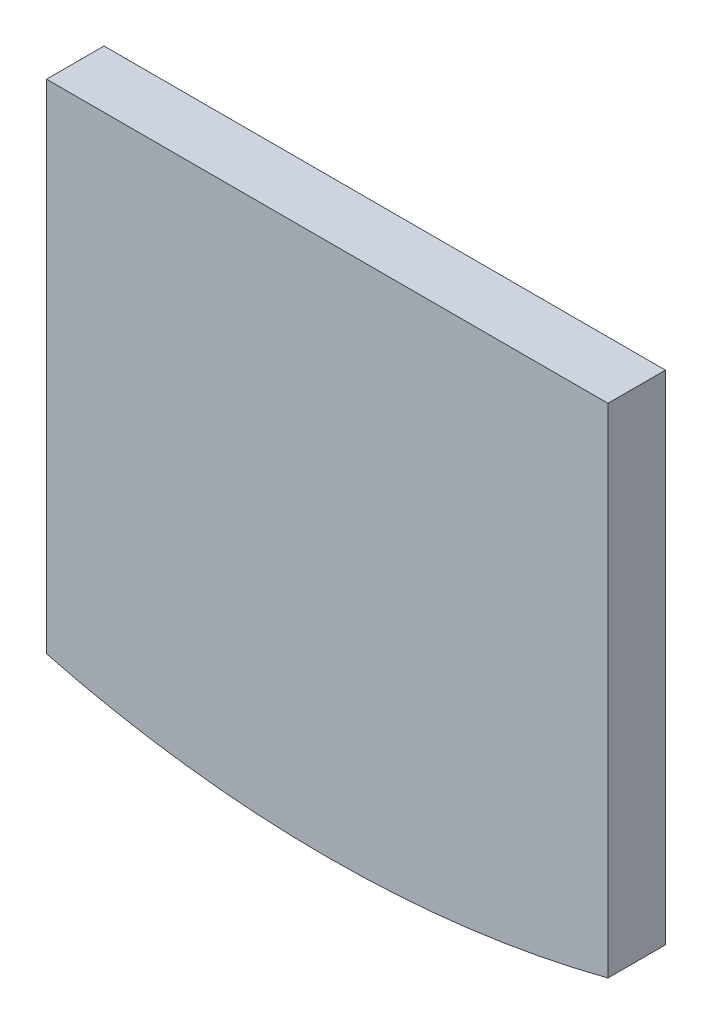
from build123d import *

# Parameters (mm, degrees)
BOSS_EXTRUDE1_DEPTH = 13


with BuildPart() as part:
    # Sketch1 → Boss-Extrude1 (new, symmetric)
    with BuildSketch(Plane.XY):
        with BuildLine():
            Line((-127, 152.4), (127, 152.4))
            Line((127, 152.4), (127, -72.768884968))
            ThreePointArc((127, -72.768884968), (0, -88.9), (-127, -72.768884968))
            Line((-127, -72.768884968), (-127, 152.4))
        make_face()
    extrude(amount=BOSS_EXTRUDE1_DEPTH, both=True)


solid = part.part
